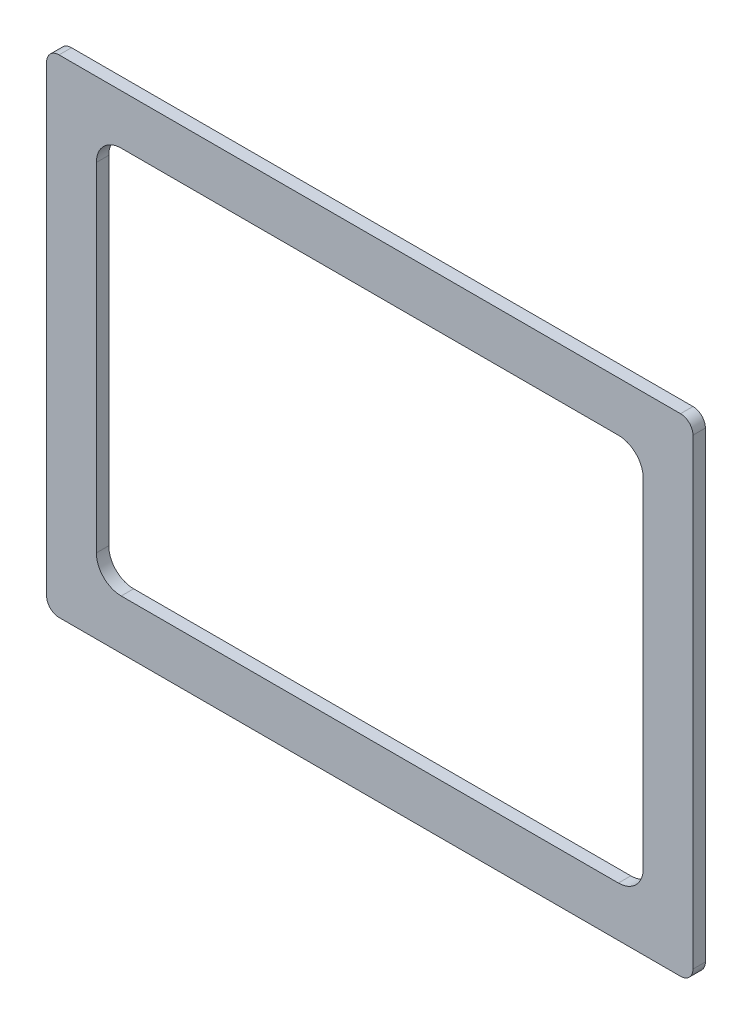
from build123d import *

# Parameters (mm, degrees)
SKETCH1_W           = 260
SKETCH1_H           = 196
SKETCH1_W_2         = 220
SKETCH1_H_2         = 156
BOSS_EXTRUDE1_DEPTH = 5
FILLET1_R           = 5
FILLET2_R           = 10


with BuildPart() as part:
    # Sketch1 → Boss-Extrude1 (new body)
    with BuildSketch(Plane.XY):
        Rectangle(SKETCH1_W, SKETCH1_H)
        Rectangle(SKETCH1_W_2, SKETCH1_H_2, mode=Mode.SUBTRACT)
    extrude(amount=BOSS_EXTRUDE1_DEPTH)

    # Fillet1
    fillet1_edges = [part.edges().sort_by_distance(p)[0] for p in [
        (-130, 98, 2.5),
        (130, 98, 2.5),
        (130, -98, 2.5),
        (-130, -98, 2.5),
    ]]
    fillet(fillet1_edges, radius=FILLET1_R)

    # Fillet2
    fillet2_edges = [part.edges().sort_by_distance(p)[0] for p in [
        (-110, 78, 2.5),
        (-110, -78, 2.5),
        (110, -78, 2.5),
        (110, 78, 2.5),
    ]]
    fillet(fillet2_edges, radius=FILLET2_R)


solid = part.part
